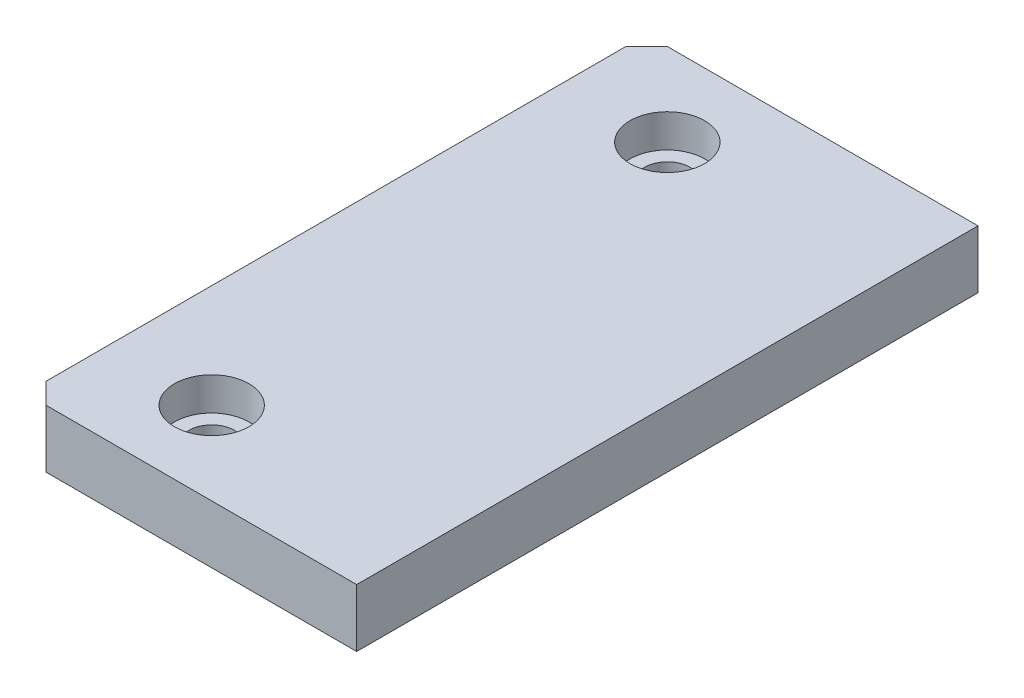
from build123d import *

# Parameters (mm, degrees)
SKETCH1_W                                           = 80
SKETCH1_H                                           = 150
BOSS_EXTRUDE1_DEPTH                                 = 14
HOLE_SIZE_BY_SOCKET_HEAD_CAP_SCREW_TYPE_D           = 11
HOLE_SIZE_BY_SOCKET_HEAD_CAP_SCREW_TYPE_CBORE_D     = 18
HOLE_SIZE_BY_SOCKET_HEAD_CAP_SCREW_TYPE_CBORE_DEPTH = 8
CHAMFER1_SIZE                                       = 5


with BuildPart() as part:
    # Sketch1 → Boss-Extrude1 (new body)
    with BuildSketch(Plane(origin=(0, 0, 0), x_dir=(1, 0, 0), z_dir=(0, 1, 0))):
        with Locations((40, 75)):
            Rectangle(SKETCH1_W, SKETCH1_H)
    extrude(amount=BOSS_EXTRUDE1_DEPTH)

    # Hole size (by socket head cap screw type)1 (through all)
    with Locations(Plane(origin=(0, 14, 0), x_dir=(1, 0, 0), z_dir=(0, 1, 0))):
        with Locations((25, 130), (25, 20)):
            CounterBoreHole(HOLE_SIZE_BY_SOCKET_HEAD_CAP_SCREW_TYPE_D / 2, HOLE_SIZE_BY_SOCKET_HEAD_CAP_SCREW_TYPE_CBORE_D / 2, HOLE_SIZE_BY_SOCKET_HEAD_CAP_SCREW_TYPE_CBORE_DEPTH)

    # Chamfer1
    chamfer1_edges = [part.edges().sort_by_distance(p)[0] for p in [
        (0, 7, -150),
        (0, 7, 0),
    ]]
    chamfer(chamfer1_edges, length=CHAMFER1_SIZE)


solid = part.part
